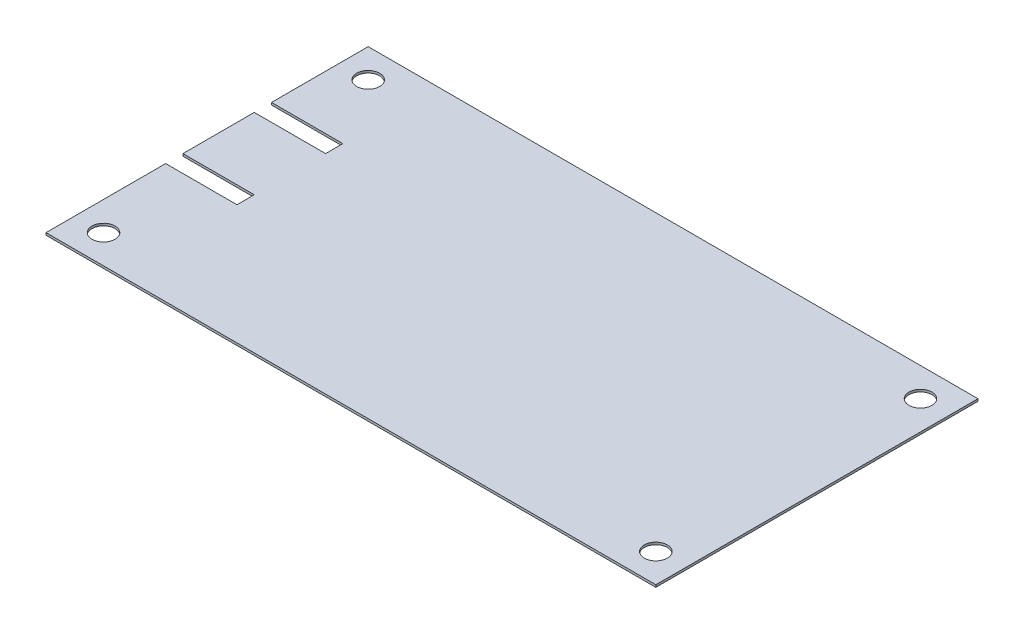
SolidWorks part; units mm, degrees
ref_plane "前视基准面" through (0, 0, 0) normal (0, 0, 1) x (1, 0, 0)
ref_plane "上视基准面" through (0, 0, 0) normal (0, 1, 0) x (1, 0, 0)
ref_plane "右视基准面" through (0, 0, 0) normal (1, 0, 0) x (0, 0, -1)
sketch "草图1" plane through (0, 0, 0) normal (0, 1, 0) x (1, 0, 0)
  line L1 (-265, -140) -> (265, -140)
  line L2 (-265, -140) -> (-265, 140)
  line L3 (-265, 140) -> (265, 140)
  line L4 (265, -140) -> (265, 140)
  line L5 (-265, -140) -> (265, 140) construction
  line L6 (-265, 140) -> (265, -140) construction
  point P0 (0, 0)
  dimension "D1" = 530
  dimension "D2" = 280
extrude "凸台-拉伸1" add sketch "草图1" along normal blind 2
sketch "草图2" plane through (0, 2, 0) normal (0, 1, 0) x (1, 0, 0)
  line L0 (-265, 140) -> (-265, -140) construction
  line L1 (-1.1, 0) -> (1.1, 0) construction
  line L2 (0, -1.1) -> (0, 1.1) construction
  circle A0 centre (-240, 115) radius 10
  circle A2 centre (-240, -115) radius 10
  circle A3 centre (240, -115) radius 10
  circle A4 centre (240, 115) radius 10
  dimension "D3" = 20
  dimension "D1" = 25
  dimension "D2" = 115
extrude "切除-拉伸1" cut sketch "草图2" against normal blind 2
sketch "草图3" plane through (0, 2, 0) normal (0, 1, 0) x (1, 0, 0)
  line L0 (-265, -140) -> (265, -140) construction
  line L1 (-299.0841, -21) -> (-203, -21)
  line L2 (-299.0841, -21) -> (-299.0841, -36)
  line L3 (-299.0841, -36) -> (-203, -36)
  line L4 (-203, -21) -> (-203, -36)
  line L5 (-296.3127, 56) -> (-203, 56)
  line L6 (-296.3127, 56) -> (-296.3127, 41)
  line L7 (-296.3127, 41) -> (-203, 41)
  line L8 (-203, 56) -> (-203, 41)
  line L9 (-265, 140) -> (-265, -140) construction
  dimension "D1" = 104
  dimension "D2" = 15
  dimension "D3" = 62
  dimension "D4" = 62
  dimension "D5" = 15
  dimension "D6" = 62
extrude "切除-拉伸2" cut sketch "草图3" against normal blind 10
